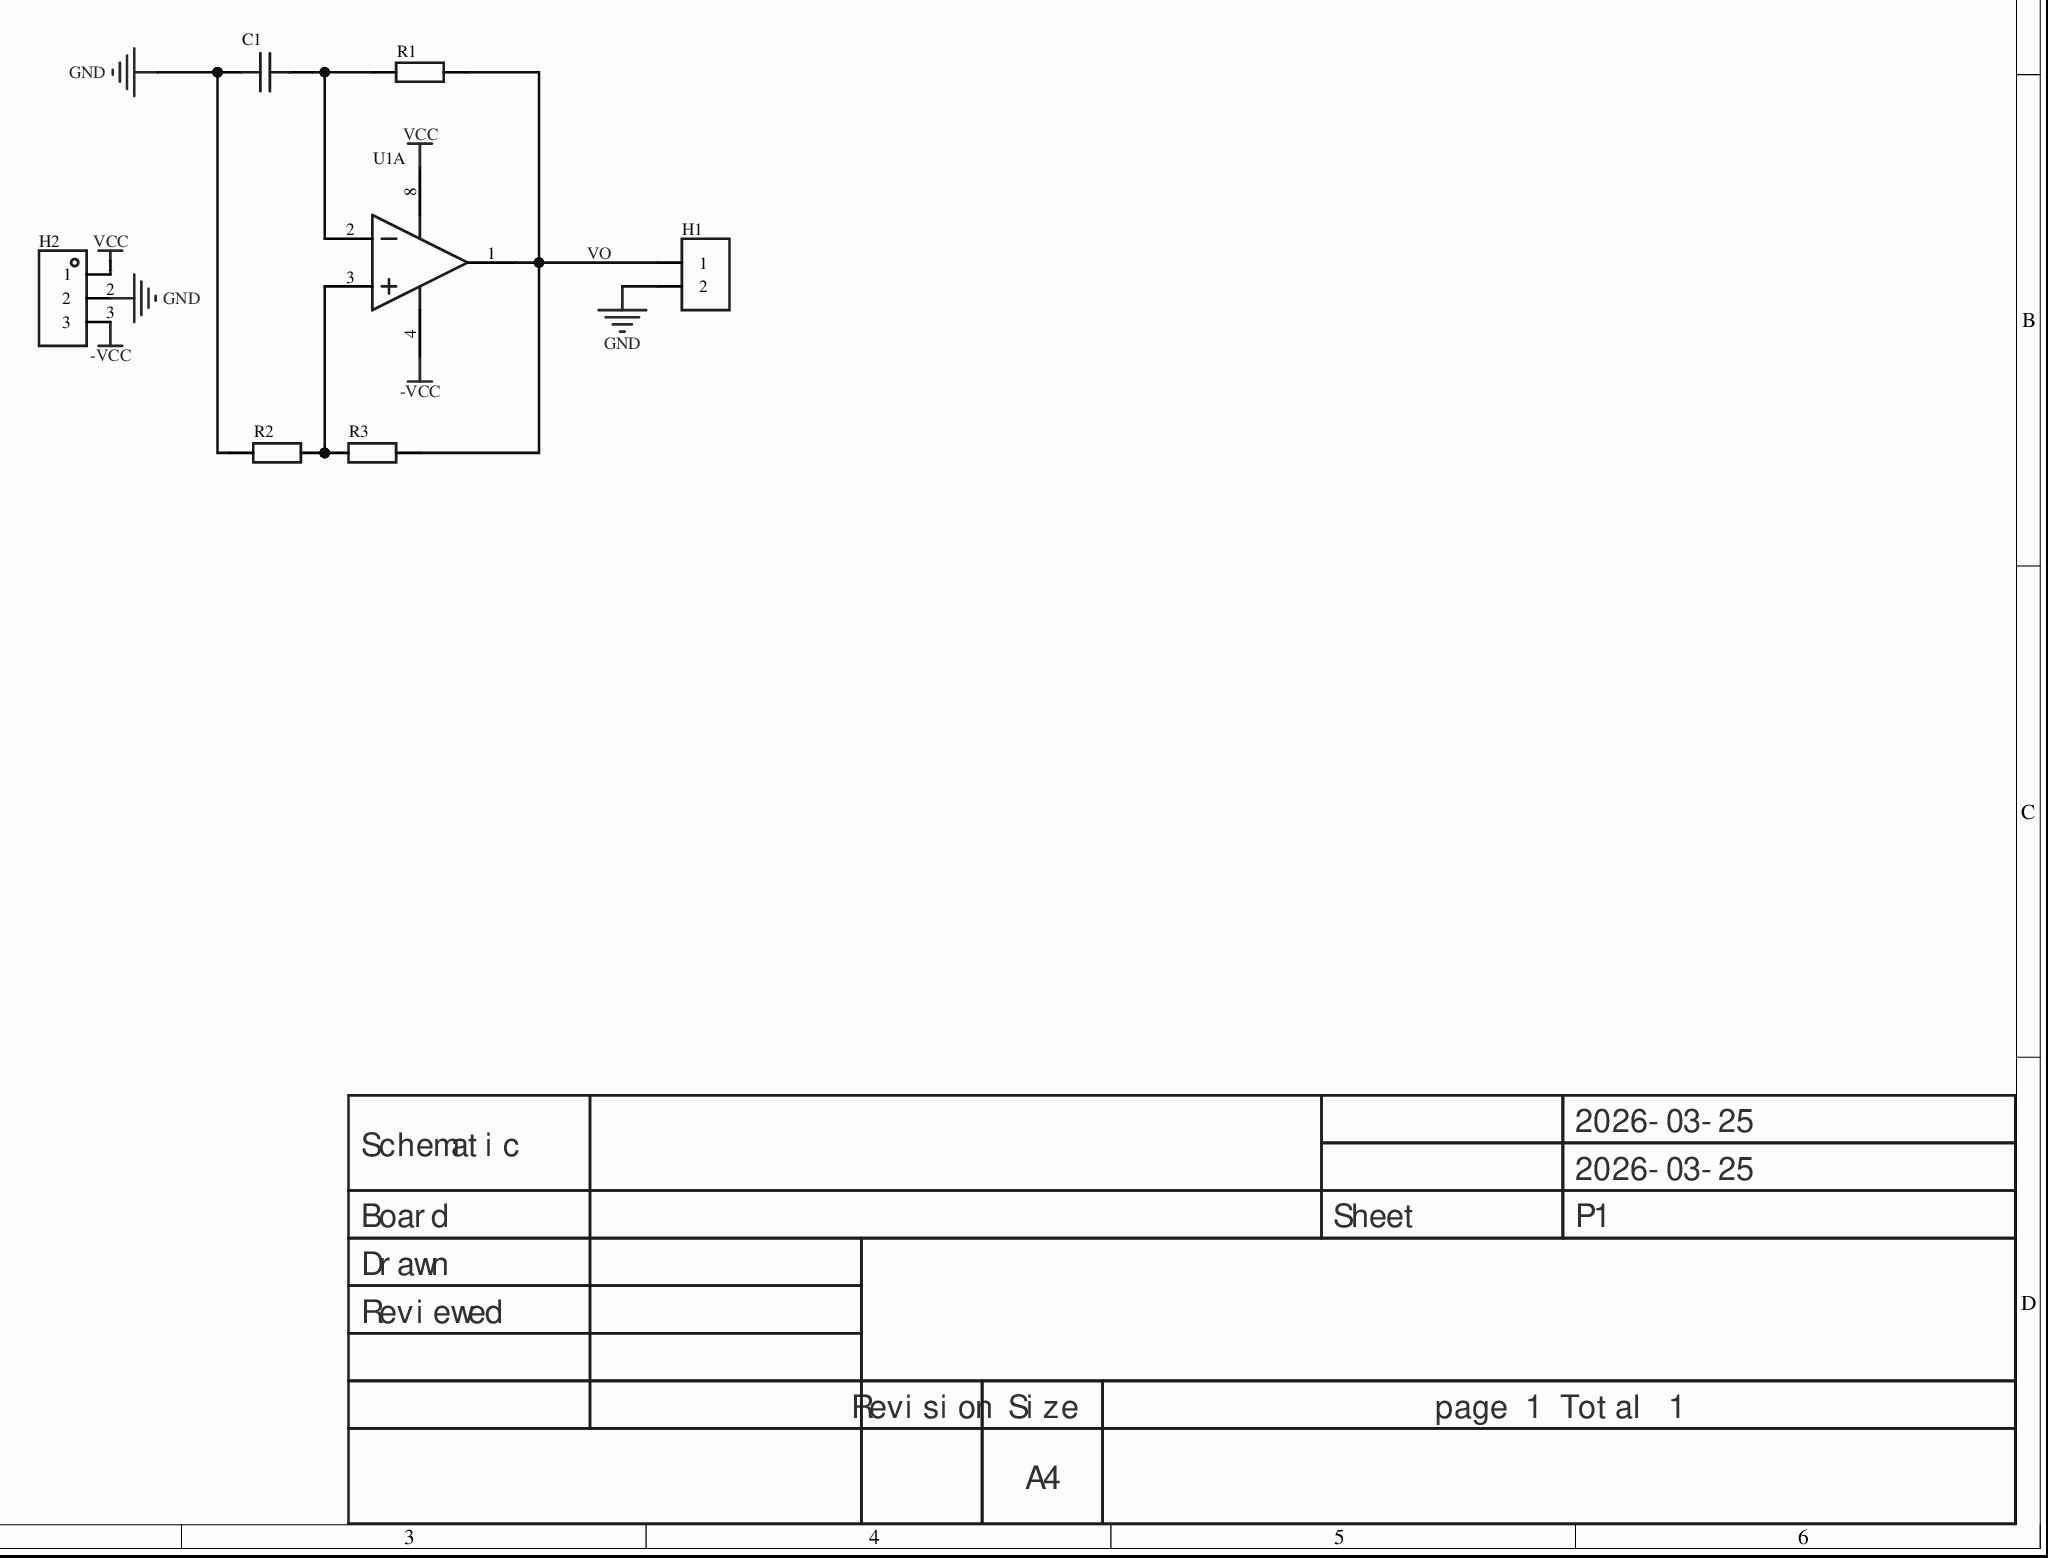
[diagram p0: MISC89039-3.schdoc]
# Altium project MISC89039-2.PrjPcb
1 sheet, 7 parts. Net scope: global (net labels, ports and power ports of the same name join across sheets).
Board file: MISC89039.pcbdoc

## Sheet MISC89039-3.schdoc
size 297 x 209 mm; Version: V1.0; @Project Name: MISC89039; @Update Date: 2026-03-25; @Create Date: 2026-03-25; @Board Name: MISC89039; @Create Time: 22:51:40; @Page Count: 1; @Page No: 1; @Schematic Name: MISC89039; @Update Time: 22:51:40; Size: A4

### Parts
C1  100nF  [C0603]  (value not drawn)
H1  (no value)  [HDR-TH_2P-P2.54-V-F]
H2  (no value)  [HDR-TH_3P-P2.54-V-M]
R1  10K  [R0603]  (value not drawn)
R2  10K  [R0603]  (value not drawn)
R3  10K  [R0603]  (value not drawn)
U1  NE5532DRG4  [SOIC-8_L5.0-W4.0-P1.27-LS6.0-BL]  (value not drawn)  (part A of 2)

### Nets
-VCC: H2.3 U1.4(VCC-)
GND: C1.1 H1.2 H2.2 R2.1
VCC: H2.1 U1.8(VCC+)
VO: H1.1 R1.2 R3.2 U1.1(OUT1)
NetC1_2: C1.2 R1.1 U1.2(IN1-)
NetR2_2: R2.2 R3.1 U1.3(IN1+)

### Notes on the sheet
- 2026-03-25
- Schematic
- Board
- Sheet
- P1
- Drawn
- Reviewed
- Revision
- Size
- A4
- page 1 Total 1

### Library data of the parts
C1 = CAP_0603: Symbol: Capacitance; ConvertToPcb: yes; ModelId: ac125912035d415993ca9572d50418b10819f05c4eef4c71ace90d822a990e87; ModelName: C0603_L1.6-W0.8-H0.8; ModelTransform: 62.992,31.496,0,0,0,0,0,0,0; Device: CAP_0603; AddInBom: yes; Supplier Footprint: 0603; FootprintName: C0603; Value: 100nF
H1 = HDR-F_2.54_1x2P: Symbol: Header-Female-2.54_1x2; ConvertToPcb: yes; ModelId: a9450ef445564560a104363b9aacde4e0819f05c4eef4c71ace90d822a990e87; ModelName: HDR-TH_2P-P2.54-F-LI-1X2P; ModelTransform: 215.7476,98.425,0,0,0,0,0,0,-129.921; Device: HDR-F_2.54_1x2P; AddInBom: yes; SupplierPart: C49661; Supplier Footprint: 插件; FootprintName: HDR-TH_2P-P2.54-V-F
H2 = HDR-M_2.54_1x3P: AddInBom: yes; ModelId: bb473b6d38ff42a99216a4fcdbdcc4cb0819f05c4eef4c71ace90d822a990e87; ModelName: HDR-TH_3P-P2.54-M-LI-1X3P; ModelTransform: 300.03877,100,0,0,0,0,0,0,-118.11; Symbol: HDR-M_2.54_1x3P; Device: HDR-M_2.54_1x3P; ConvertToPcb: yes; FootprintName: HDR-TH_3P-P2.54-V-M; SupplierPart: C2937625; Supplier Footprint: 插件
R1 = Res_0603: Symbol: Resistor; ConvertToPcb: yes; ModelId: fc143cca1e79419f9cd78b61e9279f080819f05c4eef4c71ace90d822a990e87; ModelTransform: 31.8897,63.7794,0,90,0,0,0,0,0; Device: Res_0603; AddInBom: yes; Supplier Footprint: 0603; FootprintName: R0603; ModelName: R0603; Value: 10K
R2 R3 = Res_0603: Symbol: Resistor; 3D Model: fc143cca1e79419f9cd78b61e9279f080819f05c4eef4c71ace90d822a990e87; 3D Model Transform: 31.8897,63.7794,0,90,0,0,0,0,0; ConvertToPcb: yes; Device: Res_0603; Supplier Footprint: 0603; Value: 10K; AddInBom: yes; FootprintName: R0603; ModelName: R0603
U1 = NE5532DRG4: Amplifier type: -; Output power: -;; Manufacturer: TI(德州仪器); Relevance: []; AddInBom: yes; ModelId: 7abc64c95a1a4a04a4ef38f9097c870b0819f05c4eef4c71ace90d822a990e87; ModelTransform: 192.913,236.22,0,0,0,0,0,0,0; Symbol: NE5532DRG4; Device: NE5532DRG4; LCSC Part Name: NE5532DRG4; SupplierPart: C783611; ManufacturerPart: NE5532DRG4; Supplier Footprint: SOIC-8; JLCPCB Part Class: Extended Part; Datasheet: https://www.ti.com/cn/lit/gpn/sa5532; Supplier: LCSC; ConvertToPcb: yes; FootprintName: SOIC-8_L5.0-W4.0-P1.27-LS6.0-BL; ModelName: SOIC-8_L5.0-W4.0-P1.27-LS6.0-BL; Type of Power Amplifier: -; Output Power: -